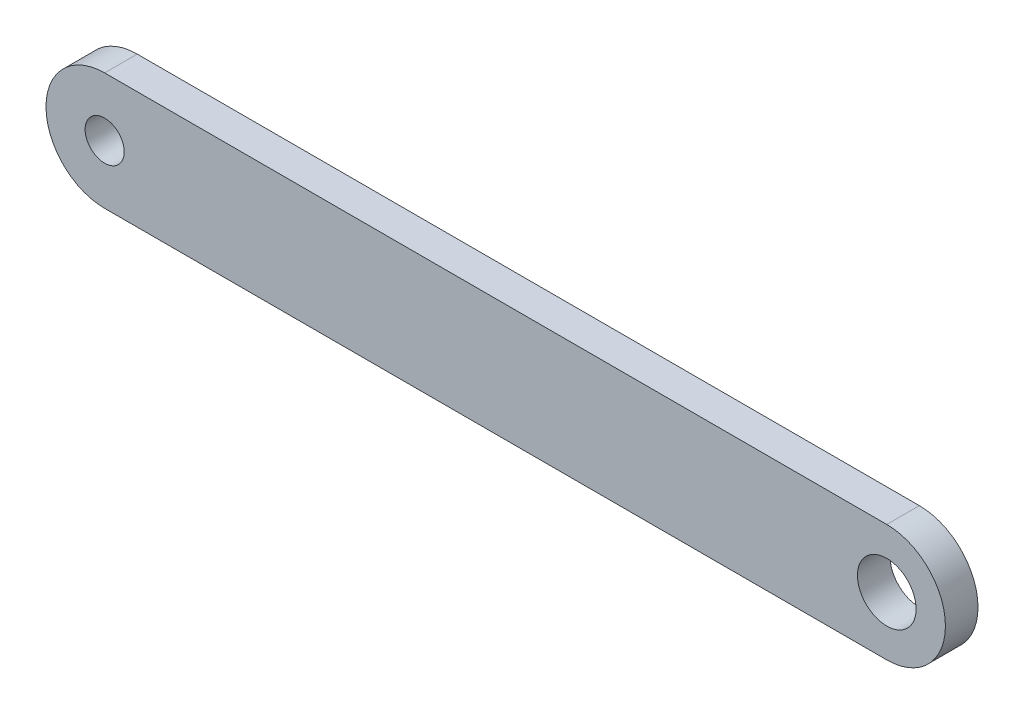
from build123d import *

# Parameters (mm, degrees)
SKETCH_1_R          = 3
EXTRUDE_1_DEPTH     = 5
SKETCH_3_R          = 6
CUT_EXTRUDE_1_DEPTH = 10
EXTRUDE_START       = -5
SKETCH_4_R          = 9
SKETCH_4_R_2        = 4.5
EXTRUDE_3_DEPTH     = 5


with BuildPart() as part:
    # 草图1 → 凸台-拉伸1 (new body)
    with BuildSketch(Plane.XY):
        with BuildLine():
            Line((0, 9), (120, 9))
            ThreePointArc((120, 9), (129, 0), (120, -9))
            Line((120, -9), (0, -9))
            ThreePointArc((0, -9), (-9, 0), (0, 9))
        make_face()
        Circle(SKETCH_1_R, mode=Mode.SUBTRACT)
        with Locations((120, 0)):
            Circle(SKETCH_1_R, mode=Mode.SUBTRACT)
    extrude(amount=EXTRUDE_1_DEPTH)

    # 草图3 → 切除-拉伸1 (cut)
    with BuildSketch(Plane.XY.offset(5)):
        with Locations((120, 0)):
            Circle(SKETCH_3_R)
    extrude(amount=-CUT_EXTRUDE_1_DEPTH, mode=Mode.SUBTRACT)

    # 草图4 → 凸台-拉伸3 (add)
    with BuildSketch(Plane.XY.offset(5).offset(EXTRUDE_START)):
        with Locations((120, 0)):
            Circle(SKETCH_4_R)
        with Locations((120, 0)):
            Circle(SKETCH_4_R_2, mode=Mode.SUBTRACT)
    extrude(amount=EXTRUDE_3_DEPTH)


solid = part.part
